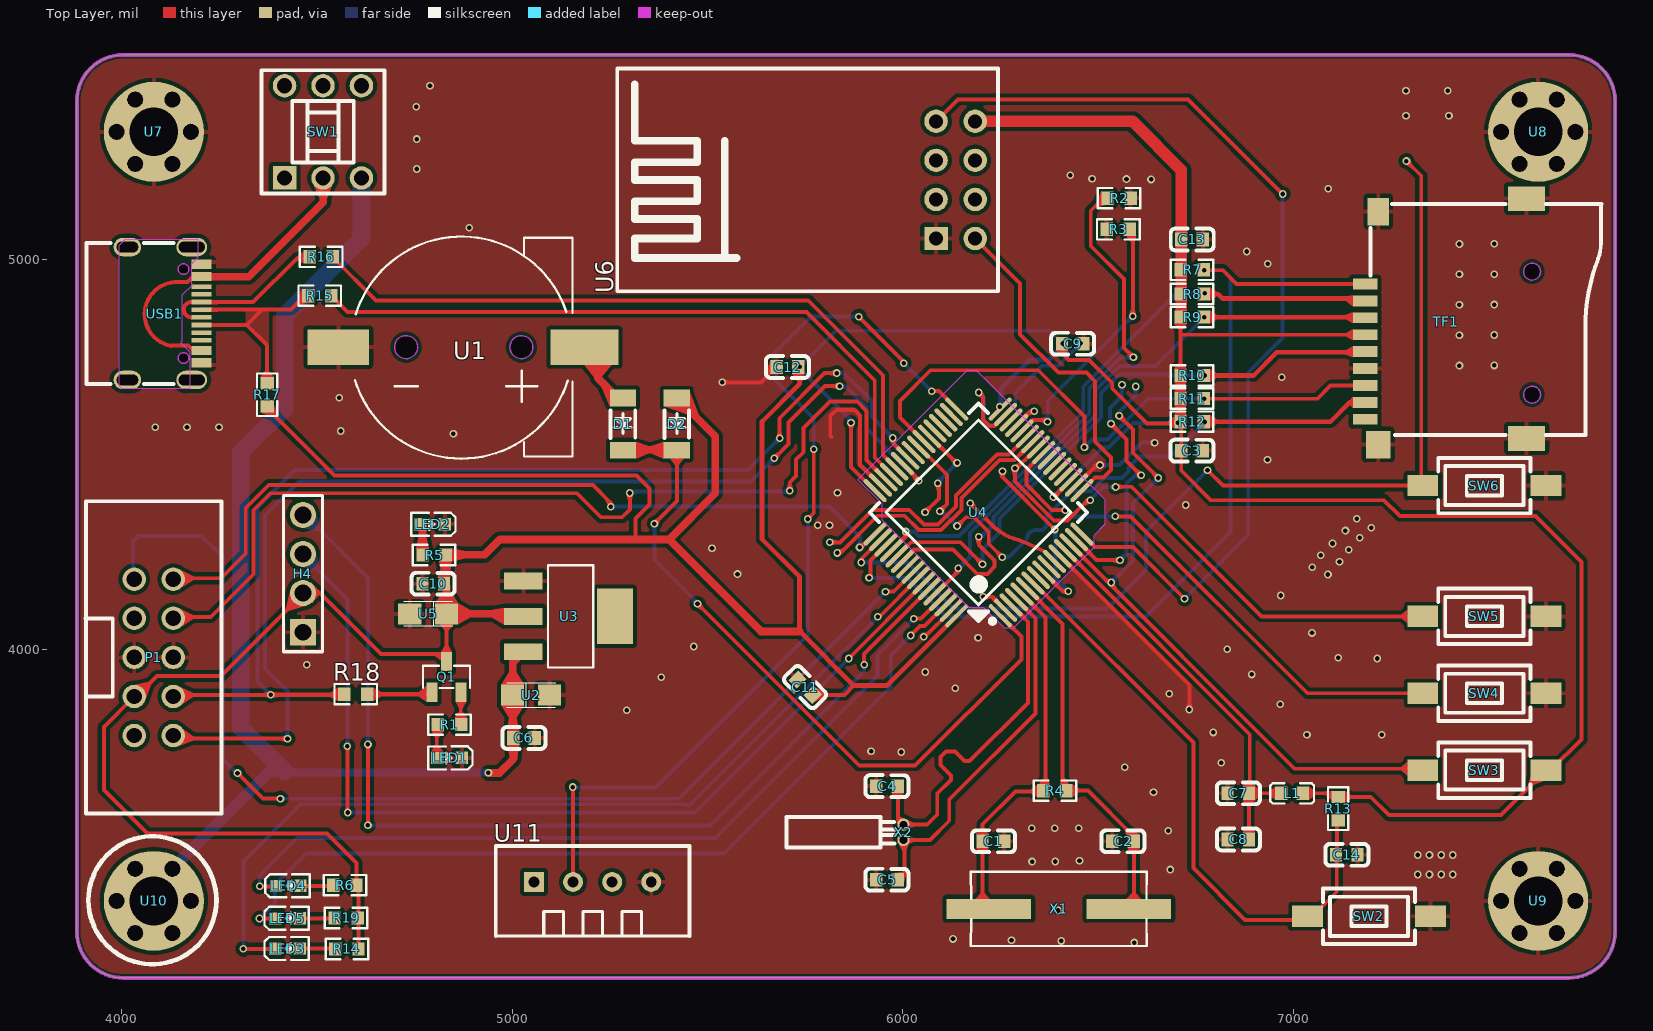
[diagram p0: Top Layer view]
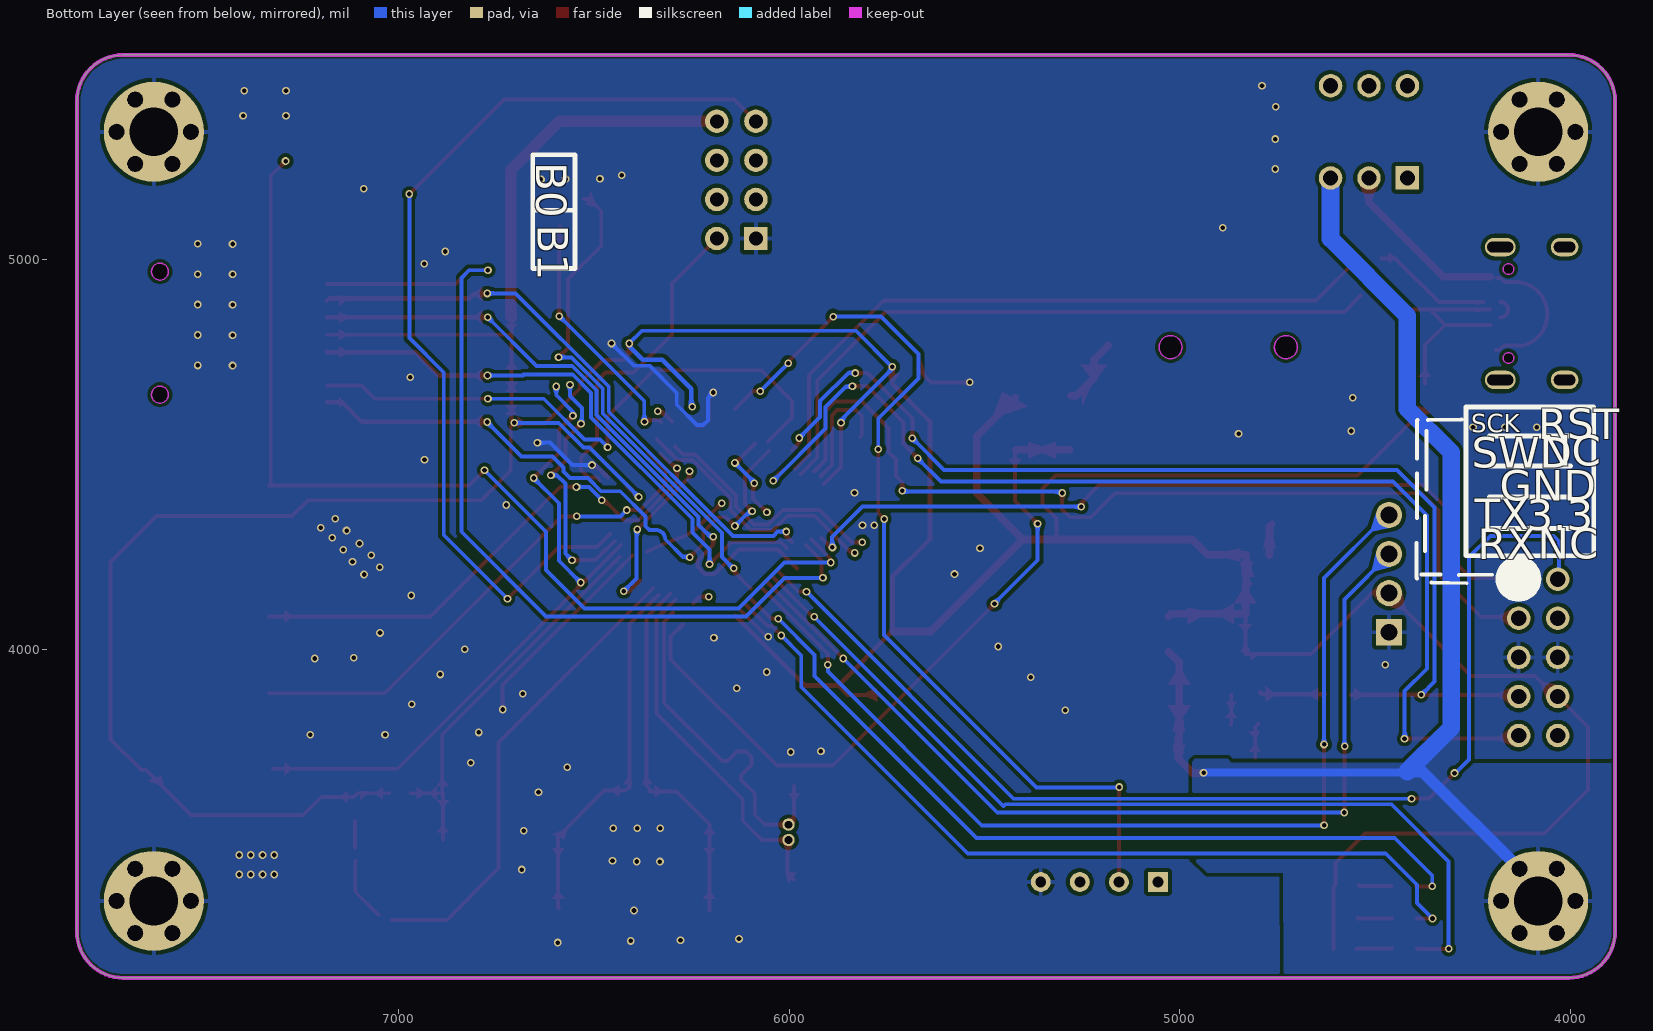
[diagram p1: Bottom Layer view, seen from below]
# Altium PCB MISC52064.pcbdoc (part 1 of 2)
Units mil, origin at the board's own origin, x right, y up, seen from the top; angles counter-clockwise.
Board outline 3937.01 x 2362.2 mil, 2 copper layers (Top Layer, Bottom Layer), stack 62.205 mil thick; 65 components, 70 nets, 266 pads, 190 vias.

## Layer stack, top to bottom
Top Solder Mask Layer: solder mask 0.394, Dk 3.3
Top Layer: signal copper 1.378
Dielectric1: surface 59.449, FR4, Dk 4.5
Bottom Layer: signal copper 1.378
Bottom Solder Mask Layer: solder mask 0.394, Dk 3.3

## Board outline
4004.35,5522.81 ccw(c4004.35,5404.7) 3886.24,5404.7 3886.24,3278.71 ccw(c4004.35,3278.71) 4004.35,3160.6 7705.14,3160.6 ccw(c7705.14,3278.71) 7823.25,3278.71 7823.25,5404.7 ccw(c7705.14,5404.7) 7705.14,5522.81 4004.35,5522.81

## Design rules (kind name [scope] priority, off if disabled: settings)
BoardOutlineClearance copperThickness2oz_1 [All] p2 off: genericclearance=7.99 ignorepadtopadclearanceinfootprint=FALSE except(0: Arc-SplitContinuation Track-SplitContinuation SMDPad-SplitContinuation THPad-SplitContinuation Via-SplitContinuation Fill-SplitContinuation Region-SplitContinuation Poly-SplitContinuation Text-SplitContinuation Hole-SplitContinuation; 5.98: SMDPad-CutoutEdge THPad-CutoutEdge Via-CutoutEdge Fill-CutoutEdge Region-CutoutEdge Text-CutoutEdge Hole-CutoutEdge; 10: Poly-OutlineEdge Poly-CutoutEdge; 11.81: Arc-OutlineEdge Track-OutlineEdge SMDPad-OutlineEdge THPad-OutlineEdge Via-OutlineEdge Fill-OutlineEdge Region-OutlineEdge Text-OutlineEdge Hole-OutlineEdge Arc-CutoutEdge Track-CutoutEdge)
BoardOutlineClearance Plane_innerPlane_1 [All] p4 off: genericclearance=4.02 ignorepadtopadclearanceinfootprint=FALSE except(0: Arc-SplitContinuation Track-SplitContinuation SMDPad-SplitContinuation THPad-SplitContinuation Via-SplitContinuation Fill-SplitContinuation Region-SplitContinuation Poly-SplitContinuation Text-SplitContinuation Hole-SplitContinuation; 5.98: SMDPad-CutoutEdge THPad-CutoutEdge Via-CutoutEdge Fill-CutoutEdge Region-CutoutEdge Text-CutoutEdge Hole-CutoutEdge; 10: Poly-OutlineEdge Poly-CutoutEdge; 11.81: Arc-OutlineEdge Track-OutlineEdge SMDPad-OutlineEdge THPad-OutlineEdge Via-OutlineEdge Fill-OutlineEdge Region-OutlineEdge Text-OutlineEdge Hole-OutlineEdge Arc-CutoutEdge Track-CutoutEdge)
BoardOutlineClearance Copper_copperRegion_1 [All] p6 off: genericclearance=4.02 ignorepadtopadclearanceinfootprint=FALSE except(0: Arc-SplitContinuation Track-SplitContinuation SMDPad-SplitContinuation THPad-SplitContinuation Via-SplitContinuation Fill-SplitContinuation Region-SplitContinuation Poly-SplitContinuation Text-SplitContinuation Hole-SplitContinuation; 5.98: SMDPad-CutoutEdge THPad-CutoutEdge Via-CutoutEdge Fill-CutoutEdge Region-CutoutEdge Text-CutoutEdge Hole-CutoutEdge; 10: Poly-OutlineEdge Poly-CutoutEdge; 11.81: Arc-OutlineEdge Track-OutlineEdge SMDPad-OutlineEdge THPad-OutlineEdge Via-OutlineEdge Fill-OutlineEdge Region-OutlineEdge Text-OutlineEdge Hole-OutlineEdge Arc-CutoutEdge Track-CutoutEdge)
BoardOutlineClearance copperThickness1oz_1 [All] p8: genericclearance=4.02 ignorepadtopadclearanceinfootprint=FALSE except(0: Arc-SplitContinuation Track-SplitContinuation SMDPad-SplitContinuation THPad-SplitContinuation Via-SplitContinuation Fill-SplitContinuation Region-SplitContinuation Poly-SplitContinuation Text-SplitContinuation Hole-SplitContinuation; 5.98: SMDPad-CutoutEdge THPad-CutoutEdge Via-CutoutEdge Fill-CutoutEdge Region-CutoutEdge Text-CutoutEdge Hole-CutoutEdge; 10: Poly-OutlineEdge Poly-CutoutEdge; 11.81: Arc-OutlineEdge Track-OutlineEdge SMDPad-OutlineEdge THPad-OutlineEdge Via-OutlineEdge Fill-OutlineEdge Region-OutlineEdge Text-OutlineEdge Hole-OutlineEdge Arc-CutoutEdge Track-CutoutEdge)
Clearance copperThickness2oz [All] p1 off: gap=7.99 ignorepadtopadclearanceinfootprint=FALSE except(5.98: SMDPad-Track SMDPad-SMDPad THPad-Track SMDPad-THPad THPad-THPad Track-Via SMDPad-Via THPad-Via Via-Via Fill-Track Region-Track Fill-SMDPad Region-SMDPad Fill-THPad Region-THPad Fill-Via Region-Via Fill-Fill Fill-Region Region-Region Arc-Track Arc-SMDPad Arc-THPad Arc-Via Fill-Arc Region-Arc Arc-Arc Text-Track SMDPad-Text Text-THPad Text-Via Fill-Text Region-Text Arc-Text Text-Text Hole-Track Hole-SMDPad Hole-THPad Hole-Via Fill-Hole Region-Hole Hole-Arc Hole-Text; 10: Poly-Track Poly-SMDPad Poly-THPad Poly-Via Poly-Fill Poly-Region Poly-Poly Poly-Arc Poly-Text Poly-Hole)
Clearance Plane_innerPlane [All] p3 off: gap=4.02 ignorepadtopadclearanceinfootprint=FALSE except(5.98: SMDPad-Track SMDPad-SMDPad THPad-Track SMDPad-THPad THPad-THPad Track-Via SMDPad-Via THPad-Via Via-Via Fill-Track Region-Track Fill-SMDPad Region-SMDPad Fill-THPad Region-THPad Fill-Via Region-Via Fill-Fill Fill-Region Region-Region Arc-Track Arc-SMDPad Arc-THPad Arc-Via Fill-Arc Region-Arc Arc-Arc Text-Track SMDPad-Text Text-THPad Text-Via Fill-Text Region-Text Arc-Text Text-Text Hole-Track Hole-SMDPad Hole-THPad Hole-Via Fill-Hole Region-Hole Hole-Arc Hole-Text; 10: Poly-Track Poly-SMDPad Poly-THPad Poly-Via Poly-Fill Poly-Region Poly-Poly Poly-Arc Poly-Text Poly-Hole)
Clearance Copper_copperRegion [All] p5 off: gap=4.02 ignorepadtopadclearanceinfootprint=FALSE except(5.98: SMDPad-Track SMDPad-SMDPad THPad-Track SMDPad-THPad THPad-THPad Track-Via SMDPad-Via THPad-Via Via-Via Fill-Track Region-Track Fill-SMDPad Region-SMDPad Fill-THPad Region-THPad Fill-Via Region-Via Fill-Fill Fill-Region Region-Region Arc-Track Arc-SMDPad Arc-THPad Arc-Via Fill-Arc Region-Arc Arc-Arc Text-Track SMDPad-Text Text-THPad Text-Via Fill-Text Region-Text Arc-Text Text-Text Hole-Track Hole-SMDPad Hole-THPad Hole-Via Fill-Hole Region-Hole Hole-Arc Hole-Text; 10: Poly-Track Poly-SMDPad Poly-THPad Poly-Via Poly-Fill Poly-Region Poly-Poly Poly-Arc Poly-Text Poly-Hole)
Clearance copperThickness1oz [All] p7: gap=4.02 ignorepadtopadclearanceinfootprint=FALSE except(5.98: SMDPad-Track SMDPad-SMDPad THPad-Track SMDPad-THPad THPad-THPad Track-Via SMDPad-Via THPad-Via Via-Via Fill-Track Region-Track Fill-SMDPad Region-SMDPad Fill-THPad Region-THPad Fill-Via Region-Via Fill-Fill Fill-Region Region-Region Arc-Track Arc-SMDPad Arc-THPad Arc-Via Fill-Arc Region-Arc Arc-Arc Text-Track SMDPad-Text Text-THPad Text-Via Fill-Text Region-Text Arc-Text Text-Text Hole-Track Hole-SMDPad Hole-THPad Hole-Via Fill-Hole Region-Hole Hole-Arc Hole-Text; 10: Poly-Track Poly-SMDPad Poly-THPad Poly-Via Poly-Fill Poly-Region Poly-Poly Poly-Arc Poly-Text Poly-Hole)
DiffPairsRouting differentialPair [All] p1: maxlimit=6 minlimit=6 mostfreqgap=6 toplayer_minwidth=5 toplayer_prefwidth=10 toplayer_maxwidth=100 toplayer_mingap=6 toplayer_prefgap=6 toplayer_maxgap=6 bottomlayer_minwidth=5 bottomlayer_prefwidth=10 bottomlayer_maxwidth=100 bottomlayer_mingap=6 bottomlayer_prefgap=6 bottomlayer_maxgap=6 maxuncoupledlength=10
HoleToHoleClearance otherClearance [All] p1: gap=11.8 allowstackedmicrovias=TRUE
Length netLength [All] p1: minlimit=0 maxlimit=0
PasteMaskExpansion pasteMaskExpansion [All] p1: expansion=0
PlaneConnect innerPlane [All] p1: planeconnectstyle=Relief reliefexpansion=20 reliefentries=4 reliefconductorwidth=10 reliefairgap=10
PolygonConnect copperRegion [All] p1: connectstyle=Relief reliefconductorwidth=10 reliefentries=4 polygonreliefangle="90 Angle" airgapwidth=10 via.connectstyle=Relief via.reliefconductorwidth=10 via.reliefentries=4 via.polygonreliefangle="90 Angle" via.airgapwidth=10
RoutingVias viaSize [All] p1: holewidth=12.01 width=24.02 viastyle="Through Hole" minholewidth=11.81 minwidth=19.68 maxholewidth=248.03 maxwidth=393.7
SolderMaskExpansion solderMaskExpansion [IsVia] p1: expansion=-1000 istentingtop=TRUE
SolderMaskExpansion solderMaskExpansion [All] p2: expansion=2.01 istentingtop=FALSE
Width copperThickness2oz_2 [All] p1 off: maxlimit=100 minlimit=8 preferedwidth=10
Width copperThickness1oz_2 [All] p2: maxlimit=100 minlimit=5 preferedwidth=10

## Components (designator, comment, footprint, x,y, rotation, side; value= is the part's Value field where it differs from the comment)
C1 "20pF" C0603 6231.9,3510.27 r180 top
C2 "20pF" C0603 6563.83,3510.06 r0 top
C3 "100nF" C0603 6740.29,4509.75 r0 top
C4 "20pF" C0603 5959.76,3651.05 r0 top
C5 "20pF" C0603 5959.76,3411.66 r0 top
C6 "100nF" C0603 5030.56,3774.43 r0 top
C7 "100pF" C0603 6858.68,3633.05 r180 top
C8 "100pF" C0603 6858.68,3514.94 r180 top
C9 "100nF" C0603 6435.2,4783.36 r0 top
C10 "100nF" C0603 4798.29,4169.19 r0 top
C11 "100nF" C0603 5750.07,3904.48 r315 top
C12 "100nF" C0603 5705.03,4723.84 r0 top
C13 "100nF" C0603 6740.57,5050.37 r180 top
C14 "1uF" C0603 7136.46,3475.57 r180 top
D1 "LL4148" LL-34_L3.5-W1.5-RD 5283.88,4577.93 r90 top
D2 "LL4148" LL-34_L3.5-W1.5-RD 5421.68,4577.93 r90 top
H4 "826629-4" HDR-TH_4P-P2.54-V-M-1 4464.82,4195.16 r90 top
L1 "1uH" L0603 6996.48,3633.05 r180 top
LED1 "KT-0603R" LED0603-RD 4840.02,3723.6 r180 top
LED2 "LTST-C191KRKT" LED0603-RD 4796.41,4321.75 r180 top
LED3 "LTST-C191KRKT" LED0603-RD 4425.18,3235.49 r0 top
LED4 "LTST-C191KRKT" LED0603-RD 4427.24,3395.81 r0 top
LED5 "LTST-C191KRKT" LED0603-RD 4425.24,3312.81 r0 top
P1 "2.54-2*5P box header" IDC-TH_10P-P2.54_C5665 4083.09,3980.7 r270 top
Q1 "S8050" SOT-23-3_L2.9-W1.3-P1.90-LS2.4-BR 4832.2,3930.92 r270 top
R1 "220Ω" R0603 4839.86,3808.72 r0 top
R2 "10kΩ" R0603 6553.61,5156.18 r180 top
R3 "10kΩ" R0603 6551.64,5076.32 r0 top
R4 "1MΩ" R0603 6389.51,3639.48 r180 top
R5 "220Ω" R0603 4800.48,4242.62 r0 top
R6 "220" R0603 4572.24,3397.81 r0 top
R7 "10kΩ" R0603 6740.57,4972.74 r180 top
R8 "10kΩ" R0603 6740.57,4910.63 r180 top
R9 "10kΩ" R0603 6740.57,4851.71 r180 top
R10 "10kΩ" R0603 6740.57,4702.31 r180 top
R11 "10kΩ" R0603 6740.57,4643.25 r180 top
R12 "10kΩ" R0603 6740.57,4584.2 r180 top
R13 "10kΩ" R0603 7114.59,3593.68 r90 top
R14 "220" R0603 4577.29,3234.43 r0 top
R15 "22Ω" R0603 4507.84,4906.58 r0 top
R16 "22Ω" R0603 4511.53,5005.9 r180 top
R17 "1.5kΩ" R0603 4373.31,4652.95 r270 top
R18 "10K" R0603 4599.96,3886.52 r0 top
R19 "220" R0603 4575.24,3313.81 r0 top
SW1 "XKB8080-Z" SW-TH_6P-L8.0-W8.0-P2.50 4516.16,5325.96 r0 top
SW2 "YTS1C0051AWG00" SW-SMD_L6.1-W3.6-LS8.0 7193.33,3318.08 r0 top
SW3 "YTS1C0051AWG00" SW-SMD_L6.1-W3.6-LS8.0 7488.61,3692.1 r0 top
SW4 "YTS1C0051AWG00" SW-SMD_L6.1-W3.6-LS8.0 7488.61,3888.95 r0 top
SW5 "YTS1C0051AWG00" SW-SMD_L6.1-W3.6-LS8.0 7488.61,4085.8 r0 top
SW6 "YTS1C0051AWG00" SW-SMD_L6.1-W3.6-LS8.0 7488.61,4420.45 r0 top
TF1 "TF_CARD_SELF" TF-SMD_TF-15-15 7390.18,4840.1 r0 top
U1 "CR1220-A" BAT-SMD_CR1220-2 4870.5,4774.78 r180 top
U2 "10uF" CASE-A_3216 5048.88,3884.42 r0 top
U3 "AMS1117-3.3" SOT-223-3_L6.5-W3.4-P2.30-LS7.0-BR 5146.09,4085.8 r180 top
U4 "STM32F103RCT6" LQFP-64_L10.0-W10.0-P0.50-LS12.0-BL 6193.84,4351.89 r45 top
U5 "10uF" CASE-A_3216 4785.34,4092.19 r180 top
U6 "ESP8266-01S" WIFIM-TH_ESP8266-01S 6135.24,5202.81 r90 top
U7 "" M3_花孔 4083.09,5325.96 r0 top
U8 "" M3_花孔 7626.4,5325.96 r0 top
U9 "" M3_花孔 7626.4,3357.45 r0 top
U10 "" M3_花孔 4083.09,3357.45 r0 top
U11 "DHT11" SENSOR-TH_DHT11 5206.24,3405.81 r0 top
USB1 "KH-TYPE-C-16P" USB-C-SMD_KH-TYPE-C-16P 4110.61,4860.9 r270 top
X1 "8MHz" HC-49S_L11.4-W4.8 6399.46,3337.01 r180 top
X2 "32.768kHz" OSC-TH_BD2.0-P0.70-D0.3 6001.74,3533.08 r0 top

## Footprints (in the part's own frame and the unit in brackets; to place one, negate y for a bottom-side part, rotate by r counter-clockwise, add the part's x,y. Pads: shape width x height; smd on the part's side, far side on the other; paste and mask are expansions set on the pad)
BAT-SMD_CR1220-2 [mm]
  rect 4.4x2.3 smd paste+0 mask+0.05: 1(-8,0)
  rect 4x2.3 smd paste+0 mask+0.05: 2(8,0)
  Board Outline Layer circle w0.003: c3.6,0 r0.75
  Board Outline Layer circle w0.003: c-3.9,0 r0.75
  Board Outline Layer region: 2.85,0 2.924,0.325 3.132,0.586 3.433,0.731 3.767,0.731 4.068,0.586 4.276,0.325 4.35,0 4.35,0 4.276,-0.325 4.068,-0.586 3.767,-0.731 3.433,-0.731 3.132,-0.586 2.924,-0.325 2.85,0
  Board Outline Layer region: 2.85,0 2.859,0.117 2.887,0.232 2.932,0.34 2.993,0.441 3.07,0.53 3.159,0.607 3.259,0.668 3.368,0.713 3.483,0.741 3.6,0.75 3.717,0.741 3.832,0.713 3.94,0.668 4.041,0.607 4.13,0.53 4.207,0.441 4.268,0.34 4.313,0.232 4.341,0.117 4.35,0 4.341,-0.117 4.313,-0.232 4.268,-0.34 4.207,-0.441 4.13,-0.53 4.041,-0.607 3.94,-0.668 3.832,-0.713 3.717,-0.741 3.6,-0.75 3.483,-0.741 3.368,-0.713 3.259,-0.668 3.159,-0.607 3.07,-0.53 2.993,-0.441 2.932,-0.34 2.887,-0.232 2.859,-0.117
  Board Outline Layer region: -4.65,0 -4.576,0.325 -4.368,0.586 -4.067,0.731 -3.733,0.731 -3.432,0.586 -3.224,0.325 -3.15,0 -3.15,0 -3.224,-0.325 -3.432,-0.586 -3.733,-0.731 -4.067,-0.731 -4.368,-0.586 -4.576,-0.325 -4.65,0
  Board Outline Layer region: -4.65,0 -4.641,0.117 -4.613,0.232 -4.568,0.34 -4.507,0.441 -4.43,0.53 -4.341,0.607 -4.24,0.668 -4.132,0.713 -4.017,0.741 -3.9,0.75 -3.783,0.741 -3.668,0.713 -3.559,0.668 -3.459,0.607 -3.37,0.53 -3.293,0.441 -3.232,0.34 -3.187,0.232 -3.159,0.117 -3.15,0 -3.159,-0.117 -3.187,-0.232 -3.232,-0.34 -3.293,-0.441 -3.37,-0.53 -3.459,-0.607 -3.559,-0.668 -3.668,-0.713 -3.783,-0.741 -3.9,-0.75 -4.017,-0.741 -4.132,-0.713 -4.24,-0.668 -4.341,-0.607 -4.43,-0.53 -4.507,-0.441 -4.568,-0.34 -4.613,-0.232 -4.641,-0.117
  Multi-Layer board cut-out: 2.85,0 2.924,0.325 3.132,0.586 3.433,0.731 3.767,0.731 4.068,0.586 4.276,0.325 4.35,0 4.35,0 4.276,-0.325 4.068,-0.586 3.767,-0.731 3.433,-0.731 3.132,-0.586 2.924,-0.325 2.85,0
  Multi-Layer board cut-out: -4.65,0 -4.576,0.325 -4.368,0.586 -4.067,0.731 -3.733,0.731 -3.432,0.586 -3.224,0.325 -3.15,0 -3.15,0 -3.224,-0.325 -3.432,-0.586 -3.733,-0.731 -4.067,-0.731 -4.368,-0.586 -4.576,-0.325 -4.65,0
  silkscreen extent -7.22,-7.19 6.92,7.25
C0603 [mm]
  rect 0.8x0.9 smd paste+0 mask+0.051: 1(-0.7,0) 2(0.7,0)
  silkscreen extent -1.41,-0.71 1.39,0.72
CASE-A_3216 [mil]
  rect 59.05x53.5 smd paste+0 mask+2: 1(-47.24,0) 2(47.24,0)
  silkscreen extent -63,-32 63,32
HC-49S_L11.4-W4.8 [mm]
  rect 5.5x1.3 smd paste+0 mask+0.051: 1(-4.553,0) 2(4.553,0)
  silkscreen extent -5.71,-2.41 5.71,2.41
HDR-TH_4P-P2.54-V-M-1 [mm]
  rect 1.7x1.7 hole 1.1 paste+0 mask+0.051: 1(-3.81,0)
  round 1.7 hole 1.1 paste+0 mask+0.051: 2(-1.27,0) 3(1.27,0) 4(3.81,0)
  silkscreen extent -5.08,-1.27 5.08,1.27
IDC-TH_10P-P2.54_C5665 [mil]
  round 60 hole 39.37 paste+0 mask+1.97: 1(-200,-50) 2(-200,50) 3(-100,-50) 4(-100,50) 5(0,-50) 6(0,50) 7(100,-50) 8(100,50) 9(200,-50) 10(200,50)
  silkscreen extent -400,-175 400,173
L0603 [mm]
  rect 0.8x0.864 smd paste-100 mask+0.051: 1(-0.7,0) 2(0.7,0)
  silkscreen extent -1.42,-0.65 1.41,0.67
LED0603-RD [mm]
  rect 0.8x0.8 smd paste+0 mask+0.051: 1(-0.799,-0.003) 2(0.799,0.003)
  silkscreen extent -1.49,-0.75 1.39,0.76
LL-34_L3.5-W1.5-RD [mm]
  rect 1.1x1.7 smd paste+0 mask+0.051: 1(-1.7,0) 2(1.7,0)
  silkscreen extent -0.9,-0.8 0.9,0.8
LQFP-64_L10.0-W10.0-P0.50-LS12.0-BL [mm]
  oval 0.3x2 smd paste+0 mask+0.051: 1(-3.75,-5.75) 2(-3.25,-5.75) 3(-2.75,-5.75) 4(-2.25,-5.75) 5(-1.75,-5.75) 6(-1.25,-5.75) 7(-0.75,-5.75) 8(-0.25,-5.75) 9(0.25,-5.75) 10(0.75,-5.75) 11(1.25,-5.75) 12(1.75,-5.75) 13(2.25,-5.75) 14(2.75,-5.75) 15(3.25,-5.75) 16(3.75,-5.75) 33(3.75,5.75) 34(3.25,5.75) 35(2.75,5.75) 36(2.25,5.75) 37(1.75,5.75) 38(1.25,5.75) 39(0.75,5.75) 40(0.25,5.75) 41(-0.25,5.75) 42(-0.75,5.75) 43(-1.25,5.75) 44(-1.75,5.75) 45(-2.25,5.75) 46(-2.75,5.75) 47(-3.25,5.75) 48(-3.75,5.75)
  oval 2x0.3 smd paste+0 mask+0.051: 17(5.75,-3.75) 18(5.75,-3.25) 19(5.75,-2.75) 20(5.75,-2.25) 21(5.75,-1.75) 22(5.75,-1.25) 23(5.75,-0.75) 24(5.75,-0.25) 25(5.75,0.25) 26(5.75,0.75) 27(5.75,1.25) 28(5.75,1.75) 29(5.75,2.25) 30(5.75,2.75) 31(5.75,3.25) 32(5.75,3.75) 49(-5.75,3.75) 50(-5.75,3.25) 51(-5.75,2.75) 52(-5.75,2.25) 53(-5.75,1.75) 54(-5.75,1.25) 55(-5.75,0.75) 56(-5.75,0.25) 57(-5.75,-0.25) 58(-5.75,-0.75) 59(-5.75,-1.25) 60(-5.75,-1.75) 61(-5.75,-2.25) 62(-5.75,-2.75) 63(-5.75,-3.25) 64(-5.75,-3.75)
  silkscreen extent -5,-5.79 5,5
M3_花孔 [mil]
  round 40 hole 40: 1(-95,0) 1(-47.5,-82.27) 1(-47.5,82.27) 1(47.5,-82.27) 1(47.5,82.27) 1(95,0)
  round 255.9 hole 125: 1(0,0)
OSC-TH_BD2.0-P0.70-D0.3 [mm]
  round 0.8 hole 0.5 paste+0 mask+0.051: 1(0,0.5) 2(0,-0.5)
  silkscreen extent -7.6,-1 -0.54,1
R0603 [mil]
  rect 31.75x34.02 smd paste-3937.01 mask+2: 1(-29.66,0) 2(29.66,0)
  silkscreen extent -55,-26 55,26
SENSOR-TH_DHT11 [mil]
  rect 51x51 hole 28: 1(-150,0)
  round 51 hole 28: 2(-50,0) 3(50,0) 4(150,0)
  silkscreen extent -248,-138 248,93
SOT-23-3_L2.9-W1.3-P1.90-LS2.4-BR [mm]
  rect 1.25x0.7 smd paste+0 mask+0.051: 1(1,-0.95) 2(1,0.95) 3(-1,0)
  silkscreen extent -0.73,-1.53 0.73,1.53
SOT-223-3_L6.5-W3.4-P2.30-LS7.0-BR [mm]
  rect 2.5x1.1 smd paste+0 mask+0.051: 1(2.97,-2.3) 2(2.97,0) 3(2.97,2.3)
  rect 2.34x3.6 smd paste+0 mask+0.051: 4(-2.97,0)
  silkscreen extent -1.57,-3.33 1.37,3.33
SW-SMD_L6.1-W3.6-LS8.0 [mm]
  rect 2x1.38 smd paste+0 mask+0.051: 1(-4,0) 2(4,0)
  silkscreen extent -3,-1.8 3,1.8
SW-TH_6P-L8.0-W8.0-P2.50 [mm]
  rect 1.524x1.524 hole 1 paste+0 mask+0.051: 1(-2.5,-3)
  round 1.524 hole 1 paste+0 mask+0.051: 2(0,-3) 3(2.5,-3) 4(-2.5,3) 5(0,3) 6(2.5,3)
  silkscreen extent -4,-4 4,4
TF-SMD_TF-15-15 [mil]
  rect 63x27.6 smd paste+0 mask+2: 1(-206.75,96.45) 2(-206.75,53.15) 3(-206.75,9.84) 4(-206.75,-33.47) 5(-206.75,-76.77) 6(-206.75,-120.08) 7(-206.75,-163.39) 8(-206.75,-206.7) 9(-206.75,-250)
  rect 63x70.87 smd paste+0 mask+2: 10(-173.17,-314.96)
  rect 94.49x62.99 smd paste+0 mask+2: 11(206.75,-299.22) 12(206.75,314.96)
  rect 55.1x70.9 smd paste+0 mask+2: 13(-173.15,281.51)
  Board Outline Layer circle w0.1: c220.53,-187.01 r21.65
  Board Outline Layer circle w0.1: c220.53,127.95 r21.65
  Board Outline Layer region: 242.18,-187.01 240.04,-196.41 234.03,-203.94 225.35,-208.12 215.71,-208.12 207.03,-203.94 201.02,-196.41 198.88,-187.01 198.88,-187.01 201.02,-177.61 207.03,-170.08 215.71,-165.9 225.35,-165.9 234.03,-170.08 240.04,-177.61 242.18,-187.01
  Board Outline Layer region: 242.18,-187.01 241.82,-190.99 240.72,-194.83 238.94,-198.41 236.53,-201.6 233.58,-204.29 230.18,-206.39 226.46,-207.84 222.53,-208.57 218.53,-208.57 214.6,-207.84 210.88,-206.39 207.48,-204.29 204.53,-201.6 202.12,-198.41 200.34,-194.83 199.24,-190.99 198.88,-187.01 199.24,-183.03 200.34,-179.19 202.12,-175.61 204.53,-172.42 207.48,-169.73 210.88,-167.63 214.6,-166.18 218.53,-165.45 222.53,-165.45 226.46,-166.18 230.18,-167.63 233.58,-169.73 236.53,-172.42 238.94,-175.61 240.72,-179.19 241.82,-183.03
  Board Outline Layer region: 242.18,127.95 240.04,118.55 234.03,111.02 225.35,106.84 215.71,106.84 207.03,111.02 201.02,118.55 198.88,127.95 198.88,127.95 201.02,137.35 207.03,144.88 215.71,149.06 225.35,149.06 234.03,144.88 240.04,137.35 242.18,127.95
  Board Outline Layer region: 242.18,127.95 241.82,123.97 240.72,120.13 238.94,116.55 236.53,113.36 233.58,110.67 230.18,108.57 226.46,107.12 222.53,106.39 218.53,106.39 214.6,107.12 210.88,108.57 207.48,110.67 204.53,113.36 202.12,116.55 200.34,120.13 199.24,123.97 198.88,127.95 199.24,131.93 200.34,135.77 202.12,139.35 204.53,142.54 207.48,145.23 210.88,147.33 214.6,148.78 218.53,149.51 222.53,149.51 226.46,148.78 230.18,147.33 233.58,145.23 236.53,142.54 238.94,139.35 240.72,135.77 241.82,131.93
  Multi-Layer board cut-out: 242.18,-187.01 240.04,-196.41 234.03,-203.94 225.35,-208.12 215.71,-208.12 207.03,-203.94 201.02,-196.41 198.88,-187.01 198.88,-187.01 201.02,-177.61 207.03,-170.08 215.71,-165.9 225.35,-165.9 234.03,-170.08 240.04,-177.61 242.18,-187.01
  Multi-Layer board cut-out: 242.18,127.95 240.04,118.55 234.03,111.02 225.35,106.84 215.71,106.84 207.03,111.02 201.02,118.55 198.88,127.95 198.88,127.95 201.02,137.35 207.03,144.88 215.71,149.06 225.35,149.06 234.03,144.88 240.04,137.35 242.18,127.95
  silkscreen extent -193,-290 398,301
USB-C-SMD_KH-TYPE-C-16P [mm]
  oval 1.2x2 hole 0.7 slot 1.7 at 90 deg paste+0 mask+0.051: 1(-4.32,1.765) 2(4.32,1.765)
  oval 1.2x1.8 hole 0.7 slot 1.4 at 90 deg paste+0 mask+0.051: 3(-4.32,-2.415) 4(4.32,-2.415)
  rect 0.3x1.3 smd paste-100 mask+0.05: A1(-3.35,2.415) A4(-2.55,2.415) A5(-1.25,2.415) A6(-0.25,2.415) A7(0.25,2.415) A8(1.25,2.415) A9(2.55,2.415) A12(3.35,2.415) B1(3.05,2.415) B4(2.25,2.415) B5(1.75,2.415) B6(0.75,2.415) B7(-0.75,2.415) B8(-1.75,2.415) B9(-2.25,2.415) B12(-3.05,2.415)
  Board Outline Layer circle w0.003: c-2.89,1.235 r0.35
  Board Outline Layer circle w0.003: c2.89,1.235 r0.35
  Board Outline Layer region: -2.89,1.585 -2.738,1.55 -2.616,1.453 -2.549,1.313 -2.549,1.157 -2.616,1.017 -2.738,0.92 -2.89,0.885 -2.89,0.885 -3.042,0.92 -3.164,1.017 -3.231,1.157 -3.231,1.313 -3.164,1.453 -3.042,1.55 -2.89,1.585
  Board Outline Layer region: -2.89,1.585 -2.812,1.576 -2.738,1.55 -2.672,1.509 -2.616,1.453 -2.575,1.387 -2.549,1.313 -2.54,1.235 -2.549,1.157 -2.575,1.083 -2.616,1.017 -2.672,0.961 -2.738,0.92 -2.812,0.894 -2.89,0.885 -2.968,0.894 -3.042,0.92 -3.108,0.961 -3.164,1.017 -3.205,1.083 -3.231,1.157 -3.24,1.235 -3.231,1.313 -3.205,1.387 -3.164,1.453 -3.108,1.509 -3.042,1.55 -2.968,1.576
  Board Outline Layer region: 2.89,1.585 3.042,1.55 3.164,1.453 3.231,1.313 3.231,1.157 3.164,1.017 3.042,0.92 2.89,0.885 2.89,0.885 2.738,0.92 2.616,1.017 2.549,1.157 2.549,1.313 2.616,1.453 2.738,1.55 2.89,1.585
  Board Outline Layer region: 2.89,1.585 2.968,1.576 3.042,1.55 3.108,1.509 3.164,1.453 3.205,1.387 3.231,1.313 3.24,1.235 3.231,1.157 3.205,1.083 3.164,1.017 3.108,0.961 3.042,0.92 2.968,0.894 2.89,0.885 2.812,0.894 2.738,0.92 2.672,0.961 2.616,1.017 2.575,1.083 2.549,1.157 2.54,1.235 2.549,1.313 2.575,1.387 2.616,1.453 2.672,1.509 2.738,1.55 2.812,1.576
  Multi-Layer board cut-out: -2.89,1.585 -2.738,1.55 -2.616,1.453 -2.549,1.313 -2.549,1.157 -2.616,1.017 -2.738,0.92 -2.89,0.885 -2.89,0.885 -3.042,0.92 -3.164,1.017 -3.231,1.157 -3.231,1.313 -3.164,1.453 -3.042,1.55 -2.89,1.585
  Multi-Layer board cut-out: 2.89,1.585 3.042,1.55 3.164,1.453 3.231,1.313 3.231,1.157 3.164,1.017 3.042,0.92 2.89,0.885 2.89,0.885 2.738,0.92 2.616,1.017 2.549,1.157 2.549,1.313 2.616,1.453 2.738,1.55 2.89,1.585
  silkscreen extent -4.57,-5.08 4.57,0.57
WIFIM-TH_ESP8266-01S [mil]
  rect 60x60 hole 36 paste+0 mask+1.97: 1(-150,50)
  round 60 hole 36 paste+0 mask+1.97: 2(-50,50) 3(50,50) 4(150,50) 5(-150,-50) 6(-50,-50) 7(50,-50) 8(150,-50)
  silkscreen extent -285,-109 285,866

## Via types
v1: diameter 19.68, hole 11.8, Top Layer to Bottom Layer, 190 vias

## Nets (pads, with @x,y where several pads share a name; then routed paths per layer and width w, separated by ;. In a path a pad name is that pad's centre, name@x,y a point inside that pad or via, vN(x,y) a via of type N, cw(c..) or ccw(c..) an arc to the next point about the centre after c; other vN are vias at no path point)
3.3V: C3.1 C9.1 C10.2 C11.2 C12.2 C13.2 D2.2 H4.2 L1.1 P1.7 Q1.3 R5.2 R6.2 R7.2 R8.2 R9.2 R10.2 R11.2 R12.2 R13.2 R14.2 R17.2 R19.2 SW3.2 TF1.4 U3.2 U4.19 U4.32 U4.48 U4.64 U5.1 U6.8 | length 13108.4
  Top Layer w10: P1.7@4033.09,3880.7 3955.24,3802.85 3955.24,3641.81 4067.24,3529.81 4526.24,3529.81 4601.9,3454.15 R6.2@4601.9,3397.81 4606.95,3392.76 R14.2@4606.95,3234.43 ; P1.7@4037.35,3879.01 4091.38,3933.05 4254.69,3933.05 H4.2@4461.18,4139.54 ; R17.2@4375.04,4616.6 4545.24,4446.41 5318.46,4446.41 5351.44,4413.43 5351.44,4371.62 5315.52,4335.7 5315.52,4282.65 ; H4.2@4478.2,4146.66 4507.07,4146.66 4664.72,3989 4832.74,3989 U5.1@4832.74,4092.19 ; C11.2@5769.56,3884.99 5850.79,3884.99 5874.43,3908.64 ; v1(5867.61,4581.36) 5867.61,4467.94 U4.48@5911.97,4423.58 ; v1(6385.63,4391.35) 6387.07,4391.35 U4.19@6414.9,4419.19 ; C9.1@6409.69,4775.42 6409.69,4756.89 6424.21,4742.37 6477.08,4742.37 6536.2,4683.25 6536.2,4669.11 6625.56,4579.75 R12.2@6701.52,4579.75 ; v1(6703.54,4580.92) 6712.73,4571.73 C3.1@6712.73,4509.75 6712.73,4459.33 6789.24,4382.81 7232.24,4382.81 7272.24,4342.81 7619.24,4342.81 7737.24,4224.81 7737.24,3771.05 7658.29,3692.1 SW3.2@7646.09,3692.1 7530.96,3576.97 7244.17,3576.97 7197.8,3623.34 R13.2@7114.59,3623.34 7104.88,3633.05 L1.1@7024.03,3633.05 ; R12.2@6710.91,4584.2 R11.2@6710.91,4643.25 R10.2@6710.91,4702.31 6710.91,4805.19 ; R9.2@6710.91,4851.71 6710.91,4805.19 ; TF1.4@7183.43,4806.63 6712.36,4806.63 6710.91,4805.19
  Top Layer w12: v1(5736.58,4724.42) 5736.58,4681.1 5639.74,4584.26 5639.74,4282.83 5735.92,4186.65 5735.92,4047.14 5874.43,3908.64 5959.39,3908.64 U4.64@6138.17,4087.42 ; C9.1@6404.78,4783.15 C9.1@6408.84,4783.15 ; C9.1@6408.34,4775.42 C9.1@6408.78,4774.98
  Top Layer w20: U3.2@5029.16,4085.8 5022.77,4092.19 4832.74,4092.19 U5.1@4832.58,4092.19 4832.58,4162.46 C10.2@4825.85,4169.19 4830.14,4173.48 R5.2@4830.14,4242.62 4830.81,4243.28 4929.55,4243.28 4968.92,4282.65 5315.52,4282.65 5401.99,4282.65 ; D2.2@5421.68,4644.86 5520.1,4546.43 5520.1,4400.76 5401.99,4282.65 ; 5735.92,4047.14 5637.5,4047.14 5401.99,4282.65
  Top Layer w30: U6.8@6185.24,5352.81 6588.24,5352.81 6713.01,5228.04 C13.2@6713.01,5050.37 6713.01,4853.81 R9.2@6710.91,4851.71
  Bottom Layer w10: v1(5867.61,4581.36) 5867.61,4587.97 5736.58,4719 v1(5736.58,4724.42) 5828.97,4816.81 6376.88,4816.81 v1(6409.69,4784.01) ; v1@6387.25,4390.31 6387.25,4393.45 6511.5,4517.7 6526.8,4517.7 6590.01,4580.9 v1@6704.49,4580.9
  Bottom Layer w12: v1@6250.84,4622.35 6250.84,4667.86 6325.28,4742.31 6374.95,4742.31 v1@6409.69,4777.04
  other v1: 6248.61,4622.01
5V: SW1.2 USB1.A4 USB1.A9 USB1.B4 USB1.B9 | length 814.9
  Top Layer w10: 4127.31,4778.07 cw(c4142.23,4859.17) 4137.79,4941.51 ; 4128.08,4778.84 4171.16,4778.84 4182.7,4767.3 USB1.B4@4190.65,4767.3 ; 4139.55,4941.09 4168.84,4941.09 4179.61,4951.86 USB1.B9@4189.3,4951.86
  Top Layer w20: USB1.B9@4205.64,4955.17 4326.12,4955.17 4516.82,5145.86 4516.82,5208 SW1.2@4515.82,5208.99
5VOUT: C6.1 SW1.3 U2.1 U3.3 U10.1 | length 3043.8
  Top Layer w20: v1(4939.54,3685.11) 4967.78,3685.11 5001.46,3718.79 5001.46,3719.44 ; 5003.79,3721.77 5003.79,3773.64 C6.1@5003,3774.43 5001.64,3775.79 U2.1@5001.64,3884.42 5001.64,3967.73 U3.3@5029.16,3995.25
  Bottom Layer w20: 4420.82,3685.72 4936.31,3685.72 v1@4937.57,3684.45
  Bottom Layer w30: U10.1@4078.02,3381.32 4078.02,3387.09 U10.1@4130.59,3439.73 4379.54,3688.6 4417.93,3688.6
  Bottom Layer w45: 4417.93,3688.6 4305.71,3800.82 4305.71,4505.27 4417.74,4617.3 4417.74,4855.28 4614.59,5052.13 SW1.3@4614.59,5207.85
$1N4980: D1.2 U1.1 | length 175.8
  Top Layer w20: U1.1@5183.91,4778.7 5219.68,4742.94 5219.68,4695.99 5265.51,4650.16 D1.2@5278.92,4650.16
$1N6590: D1.1 D2.1 U4.1 | length 1816.2
  Top Layer w10: v1@5364.27,4323.1 5422,4380.83 D2.1@5422,4513.51 ; v1(5474.56,4118.05) 5888.54,3704.06 6031.62,3704.06 6303.42,3975.85 6303.42,4033.77 U4.1@6272.19,4064.99
  Top Layer w20: D1.1@5282.24,4512.11 5420.02,4512.11 D2.1@5420.35,4511.78
  Bottom Layer w10: v1(5364.43,4323.03) 5364.43,4229.25 v1@5473.92,4119.76
$1N7223: C7.1 C8.1 L1.2 U4.13 | length 993.8
  Top Layer w10: U4.13@6434.33,4237.24 6888.22,3783.36 C7.1@6888.22,3633.05 ; C8.1@6886.24,3514.94 C7.1@6886.24,3633.05 C7.1@6888.22,3633.05 ; C7.1@6888.22,3632.21 C7.1@6888.22,3633.05 ; L1.2@6968.92,3633.05 C7.1@6888.22,3633.05
$1N118678: LED3.2 R14.1 | length 91.5
  Top Layer w10: LED3.2@4456.66,3235.62 4546.44,3235.62 R14.1@4547.63,3234.43
$1N123092: LED2.2 R5.1 | length 81.4
  Top Layer w20: LED2.2@4764.94,4321.61 4770.82,4315.73 R5.1@4770.82,4242.62
$1N170341: Q1.2 R1.2 | length 78
  Top Layer w10: Q1.2@4868.81,3886.43 4868.81,3809.33 R1.2@4869.52,3808.72
$1N170394: LED1.2 R1.1 | length 90.3
  Top Layer w10: R1.1@4798.84,3811.28 4807.27,3802.85 LED1.2@4807.27,3724.46
$1N175343: Q1.1 R18.2 | length 167.3
  Top Layer w12: R18.2@4629.62,3886.52 4789.77,3886.52 Q1.1@4794.8,3891.55
$1N179036: LED4.2 R6.1 | length 84.6
  Top Layer w10: LED4.2@4458.72,3395.94 4540.72,3395.94 R6.1@4542.58,3397.81
$1N179039: LED5.2 R19.1 | length 89.2
  Top Layer w10: LED5.2@4456.72,3312.94 4544.72,3312.94 R19.1@4545.58,3313.81
BOOT0: R2.2 U4.60 | length 1296.6
  Top Layer w10: U4.60@6098.57,4157.51 6143.74,4202.69 6143.74,4209.09 6142.14,4209.09 v1@6142,4209.23 ; R2.2@6519.87,5153.11 R2.2@6519.87,5154.28 ; R2.2@6525.86,5154.28 R2.2@6519.87,5154.28 ; v1@6590.09,4749.16 6566.25,4773 6566.25,4948.92 6481.29,5033.88 6481.29,5123.84 6511.72,5154.28 R2.2@6519.87,5154.28
  Bottom Layer w10: v1@6141.53,4208.61 6143.32,4208.61 6172.28,4237.57 6172.28,4299.77 6477.3,4604.79 6477.3,4668.51 6557.41,4748.62 v1(6590.44,4748.62)
  other v1: 6142.43,4209.27
BOOT1: R3.2 U4.28 | length 642.7
  Top Layer w10: U4.28@6328.14,4583.62 6333.03,4588.5 6365.98,4588.5 v1(6370.5,4583.98) ; R3.2@6581.33,5076.63 R3.2@6586.93,5076.63 ; R3.2@6586.93,5083.25 R3.2@6586.93,5076.63 ; v1@6588.9,4853.98 6588.9,5074.66 R3.2@6586.93,5076.63
  Bottom Layer w10: v1(6370.5,4583.98) 6371.07,4584.55 6371.07,4636.67 6588.18,4853.78 v1(6588.91,4853.78)
D+: R15.1 R17.1 USB1.A6 USB1.B6 | length 628.9
  Top Layer w10: USB1.B6@4205.69,4831.37 4321.06,4831.37 ; USB1.A6@4206.19,4870.68 4360.36,4870.68 ; R17.1@4372.67,4681.29 4372.67,4779.76 4321.06,4831.37 ; R15.1@4475.71,4911.66 4434.73,4870.68 4360.36,4870.68 ; 4321.06,4831.37 4360.36,4870.68
D-: R16.2 USB1.A7 USB1.B7 | length 370.2
  Top Layer w10: 4179.9,4851.06 cw(c4179.9,4870.75) 4179.9,4890.43 ; USB1.B7@4223.11,4889.82 4337.02,4889.82 4449.16,5001.96 4482.79,5001.96 R16.2@4484.36,5003.54
GND: C1.1 C2.1 C3.2 C4.1 C5.1 C6.2 C7.2 C8.2 C9.2 C10.1 C11.1 C12.1 C13.1 C14.1 H4.1 LED1.1 LED2.1 P1.5 P1.6 R2.1 R3.1 SW2.2 SW4.2 SW5.2 SW6.2 TF1.6 TF1.10 TF1.11 TF1.12 TF1.13 U1.2 U2.2 U3.1 U4.12 U4.18 U4.31 U4.47 U4.63 U5.2 U6.1 U7.1 U8.1 U9.1 U11.4 USB1.A1 USB1.A12 USB1.B1 USB1.B12 | length 1860.7
  Top Layer w10: v1@5537.55,4684.78 5637.37,4684.78 C12.1@5670.83,4718.24 ; 5818.25,4544.95 5814.36,4548.84 5814.36,4598.07 5829.91,4613.62 5877.42,4613.62 5890.81,4600.23 5890.81,4473.25 U4.47@5920.61,4443.45 ; v1(6053.47,4033.59) 6056.49,4033.59 U4.63@6124.25,4101.34 ; v1@6195.34,4657.67 6205.34,4647.67 6205.34,4589.31 6221.61,4573.04 6234.47,4573.04 U4.31@6244.24,4582.81 ; U4.12@6401.9,4241.54 6733.59,3909.85 v1(6733.59,3847.39) ; U4.18@6464.14,4441.12 6495.46,4472.44 v1@6503.1,4472.44
  Bottom Layer w10: v1(6194.69,4658.65) 6208.27,4645.07 6208.27,4587.35 6220.37,4575.26 6235.91,4575.26 6288.03,4627.38 6288.03,4657.61 6357.71,4727.29 6398.03,4727.29 v1(6455.04,4784.3) ; v1(6504.73,4472.91) 6554.58,4472.91 6612.06,4530.39 6641.9,4530.39 v1@6643.86,4528.42
  other v1: 6592.26,3250.77 6405.95,3255.02 6278.34,3256.72 6128.61,3260.13 6397.25,3332.96 7318.04,3425.01 7348.04,3425.01 7378.04,3425.01 7408.04,3425.01 6684.72,3437.65 6330.99,3458.09 6390.46,3458.33 6452.43,3459.86 7318.04,3475.01 7348.04,3475.01 7378.04,3475.01 7408.04,3475.01 6679.49,3536.83 6329.98,3543.1 6388.89,3543.78 6450.35,3543.54 6641.68,3635.37 6567.9,3699.93 6814.87,3711.24 5996.01,3738.59 5918.92,3740.54 7034.42,3782.68 7226.32,3782.74 6794.84,3788.72 5293.93,3845.13 6966,3860.58 6682.12,3887.59 6134.32,3901.88 5381.83,3929.64 6893.26,3937.14 6057.79,3943.22 4474.49,3961.53 7214.84,3977.98 7114.77,3979.98 6830.8,4001.69 5465.2,4008.47 6192.83,4031.3 7047.35,4043.39 6967.83,4139.1 7088.22,4192.93 5576.93,4193.93 7047.93,4211.71 7117.96,4225.57 7070.05,4242.34 7141.53,4255.88 5511.71,4260.28 7099.83,4272.11 7169.89,4287.07 7133.01,4305.29 7199.2,4312.26 5782.3,4318.67 5812.41,4318.61 7162.22,4335.58 6724.13,4370.69 5832.9,4402.2 6933.48,4486.22 6644.51,4529.73 4849.93,4552.99 4561.5,4560.12 4086.47,4569.39 4168.18,4569.39 4249.89,4569.39 4557.96,4644.92 5537.84,4684.73 6970.06,4698.05 7424.76,4727.6 7514.29,4728.05 7424.76,4805.42 7514.29,4805.88 7424.76,4883.24 7514.29,4883.7 7424.76,4961.06 7514.29,4961.52 6934.33,4988.15 6880.74,5019.63 7424.76,5038.89 7514.29,5039.35 4890.77,5080.41 7088.71,5179.87 6635.62,5204.04 6572.61,5204.96 6484.54,5205.54 6428.73,5214.78 4756.07,5230.61 4756.07,5307.38 7287.98,5366.74 7397.94,5366.74 4755.09,5389.98 7287.98,5431.02 7394.95,5431.02 4790.08,5443.43
JTDO: U4.55
NJTRST: P1.1 U4.56 | length 2921
  Top Layer w10: v1(4297.22,3684.63) 4362.62,3619.23 v1(4407.16,3619.23) ; v1(5955.86,4148.86) 5976.9,4148.86 U4.56@6026.82,4198.78
  Bottom Layer w10: P1.1@4030.28,4181.53 4030.28,4277.88 4044.3,4291.9 4205.67,4291.9 4260.26,4237.31 4260.26,3719.38 4295.01,3684.63 v1(4297.22,3684.63) ; v1(4407.16,3619.23) 4407.4,3618.98 5425.98,3618.98 v1(5955.86,4148.86)
PA0: SW3.1 U4.14 | length 1740.4
  Top Layer w10: U4.14@6430.11,4268.49 7003,3695.6 SW3.1@7320.92,3695.6 ; v1(6553.71,4599.24) 6589.42,4563.53 6589.42,4504.48 v1@6654.1,4439.8
  Bottom Layer w10: v1(6533.9,4172.51) 6533.9,4172.61 6589.46,4228.18 6589.46,4375.16 v1@6654.17,4439.86 ; v1@6553.46,4597.73 6553.46,4609.1 6596.27,4651.91 v1(6596.27,4674.12)
  other v1: 6654.19,4439.81
PA1: U4.15 | length 658.7
  Top Layer w10: U4.15@6446.57,4278.85 6495.71,4229.71 v1@6557.76,4229.71 ; v1(6533.13,4578.35) 6572.97,4538.5 6572.97,4483.64 v1(6609.98,4446.62)
  Bottom Layer w10: v1@6532.89,4577.34 6532.89,4580.94 6530.42,4583.41 6530.42,4619.08 6561.22,4649.88 v1(6561.22,4678.36) ; v1(6556.03,4229.58) 6573.13,4246.67 6573.13,4425.81 6593.94,4446.62 v1(6609.98,4446.62)
PA2: U4.16 U6.4 | length 2481.9
  Top Layer w10: U6.4@6085.24,5352.81 6141.24,5408.81 6730.24,5408.81 v1(6972.24,5166.81) ; U4.16@6458.31,4296.22 6491.71,4262.81 6589.24,4262.81 v1(6721.24,4130.81)
  Bottom Layer w10: v1(6721.24,4130.81) 6884.24,4293.81 6884.24,4709.81 6972.24,4797.81 v1(6972.24,5166.81)
PA3: U4.17 U6.5 | length 837.9
  Top Layer w10: U6.5@6185.24,5052.81 6300.35,4937.7 6300.35,4807.5 6398.21,4709.64 6470.22,4709.64 6492.35,4687.5 6492.35,4533.73 6533.28,4492.81 6533.28,4460.74 6513.72,4441.18 6492.35,4441.18 U4.17@6484.95,4433.78
PA4: U4.20
PA5: U4.21
PA6: U4.22
PA7: U4.23
PA8: U4.41
PA9: P1.8 R18.1 U4.42 | length 2855.4
  Top Layer w10: P1.8@4127.47,3884.84 v1(4382.74,3884.84) ; v1@4382.87,3884.69 v1@4383.23,3884.33 ; v1@5684.45,4542.3 5684.45,4592.7 5800.14,4708.39 v1(5830.95,4708.39) ; v1(5974.74,4542.15) 5974.74,4530 U4.42@5993.47,4511.27
  Top Layer w12: v1(4382.74,3884.84) R18.1@4561.13,3884.84
  Bottom Layer w10: v1@4382.3,3884.6 4348.17,3918.73 4348.17,4364.12 4444,4459.95 5603.44,4459.95 v1(5685.29,4541.79) ; v1@5834.18,4708.83 5848.69,4708.83 5920.96,4636.56 5920.96,4595.93 v1(5974.74,4542.15)
PA10: P1.10 U4.43 | length 2895.5
  Top Layer w10: P1.10@4136.19,3775.9 4139.37,3772.73 v1(4425.23,3772.73) ; v1@5673.63,4492.11 5673.63,4492.76 5707.99,4527.12 5707.99,4582.13 5800.91,4675.05 v1(5838.34,4675.05) ; U4.43@6016.54,4458.95 6040.88,4434.6 v1(6040.88,4432.66)
  Bottom Layer w10: v1@4424.87,3771.39 4424.87,3894.75 4367.87,3951.74 4367.87,4344.03 4454.74,4430.91 5611.9,4430.91 v1(5671.37,4490.38) ; v1@5837.88,4673.82 5854.96,4673.82 5906.96,4621.82 5906.96,4566.59 v1(6040.88,4432.66)
PA11: R16.1 U4.44 | length 1788.7
  Top Layer w10: R16.1@4541.19,5005.9 4541.19,5004.76 4652.14,4893.81 5758.24,4893.81 5949.24,4702.81 5949.24,4499.04 U4.44@5985.05,4463.23
PA12: R15.2 U4.45 | length 1738.8
  Top Layer w10: R15.2@4537.5,4906.58 4579.27,4864.81 5753.24,4864.81 5928.24,4689.81 5928.24,4492.21 U4.45@5971.14,4449.32
PA13: P1.4 U4.46 | length 2425.1
  Top Layer w10: P1.4@4136.1,4084.06 4228.87,4084.06 4338.34,4193.53 4338.34,4357.3 4381.92,4400.88 5166.53,4400.88 5227.94,4339.47 5281.18,4339.47 5301.39,4359.68 5301.39,4401.3 v1@5299.7,4402.99 ; v1(5710.74,4407.23) 5710.74,4428.58 5726.7,4444.54 5726.7,4486.97 5745.6,4505.88 5745.6,4568.18 5813.39,4635.97 5883.13,4635.97 ; 5883.45,4635.36 5907.17,4611.64 5907.17,4485.75 U4.46@5936.77,4456.14
  Bottom Layer w10: v1(5301.21,4401.43) 5304.85,4405.08 5710.31,4405.08 v1@5711.69,4406.46